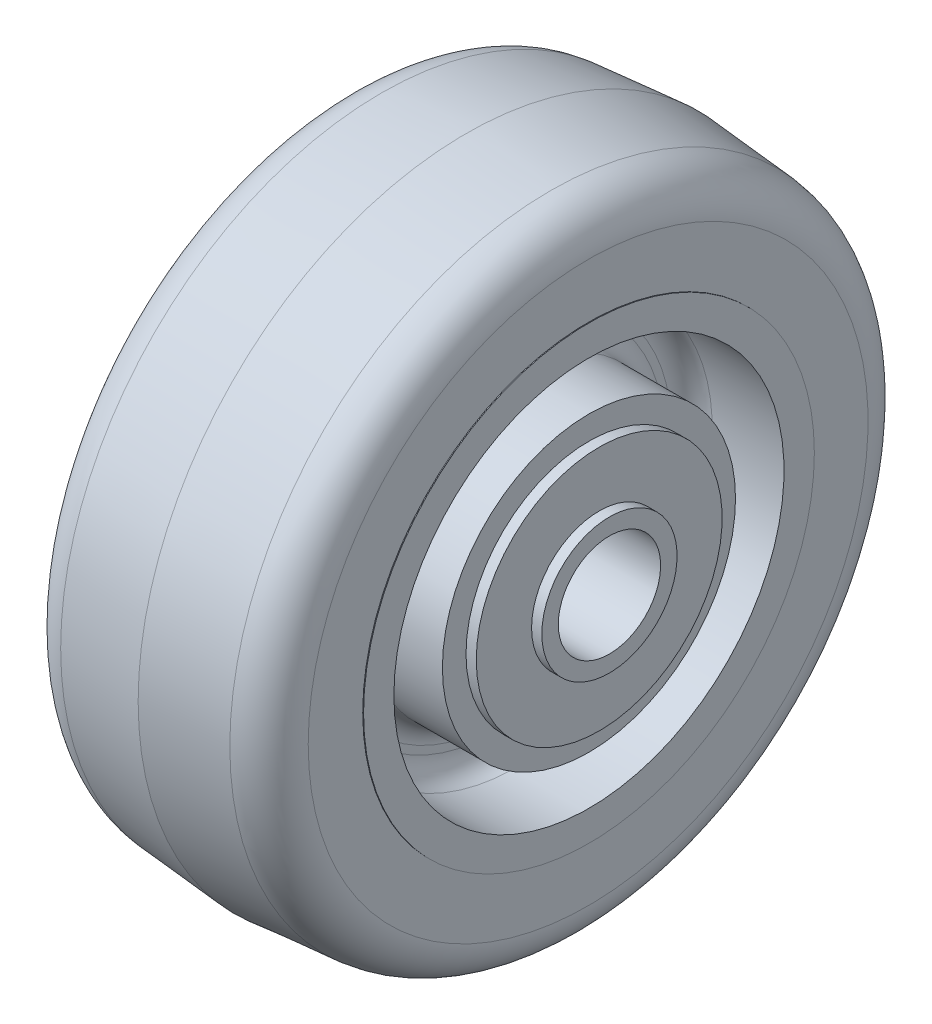
from build123d import *


with BuildPart() as part:
    # Sketch3 → Revolve1 (revolve)
    with BuildSketch(Plane.XY, mode=Mode.PRIVATE) as revolve1_sk:
        with BuildLine():
            Line((-22.225, 7.9248), (-9.525, 7.9248))
            Line((-9.525, 7.9248), (-9.525, 12.7))
            Line((-9.525, 12.7), (9.525, 12.7))
            Line((9.525, 12.7), (9.525, 7.9248))
            Line((9.525, 7.9248), (22.225, 7.9248))
            Line((22.225, 7.9248), (22.225, 10.4775))
            Line((22.225, 10.4775), (20.6375, 10.4775))
            Line((20.6375, 10.4775), (20.6375, 19.05))
            Line((20.6375, 19.05), (19.05, 19.05))
            Line((19.05, 19.05), (19.05, 22.7076))
            Line((19.05, 22.7076), (7.9375, 22.7076))
            ThreePointArc((7.9375, 22.7076), (5.69243597, 23.63753597), (4.7625, 25.8826))
            Line((4.7625, 25.8826), (4.7625, 27.051))
            ThreePointArc((4.7625, 27.051), (5.69243597, 29.29606403), (7.9375, 30.226))
            Line((7.9375, 30.226), (19.05, 30.226))
            Line((19.05, 30.226), (19.05, 34.925))
            Line((19.05, 34.925), (18.923, 34.925))
            Line((18.923, 34.925), (18.923, 43.372520863))
            ThreePointArc((18.923, 43.372520863), (17.247110014, 47.670799073), (13.104040763, 49.70027684))
            Line((13.104040763, 49.70027684), (0, 50.8))
            Line((0, 50.8), (-13.104040763, 49.70027684))
            ThreePointArc((-13.104040763, 49.70027684), (-17.247110014, 47.670799073), (-18.923, 43.372520863))
            Line((-18.923, 43.372520863), (-18.923, 34.925))
            Line((-18.923, 34.925), (-19.05, 34.925))
            Line((-19.05, 34.925), (-19.05, 30.226))
            Line((-19.05, 30.226), (-7.9375, 30.226))
            ThreePointArc((-7.9375, 30.226), (-5.69243597, 29.29606403), (-4.7625, 27.051))
            Line((-4.7625, 27.051), (-4.7625, 25.8826))
            ThreePointArc((-4.7625, 25.8826), (-5.69243597, 23.63753597), (-7.9375, 22.7076))
            Line((-7.9375, 22.7076), (-19.05, 22.7076))
            Line((-19.05, 22.7076), (-19.05, 19.05))
            Line((-19.05, 19.05), (-20.6375, 19.05))
            Line((-20.6375, 19.05), (-20.6375, 10.4775))
            Line((-20.6375, 10.4775), (-22.225, 10.4775))
            Line((-22.225, 10.4775), (-22.225, 7.9248))
        make_face()
    revolve(revolve1_sk.sketch.rotate(Axis((-32.006619827, 0, 0), (1, 0, 0)), 90), axis=Axis((-32.006619827, 0, 0), (1, 0, 0)))


solid = part.part
